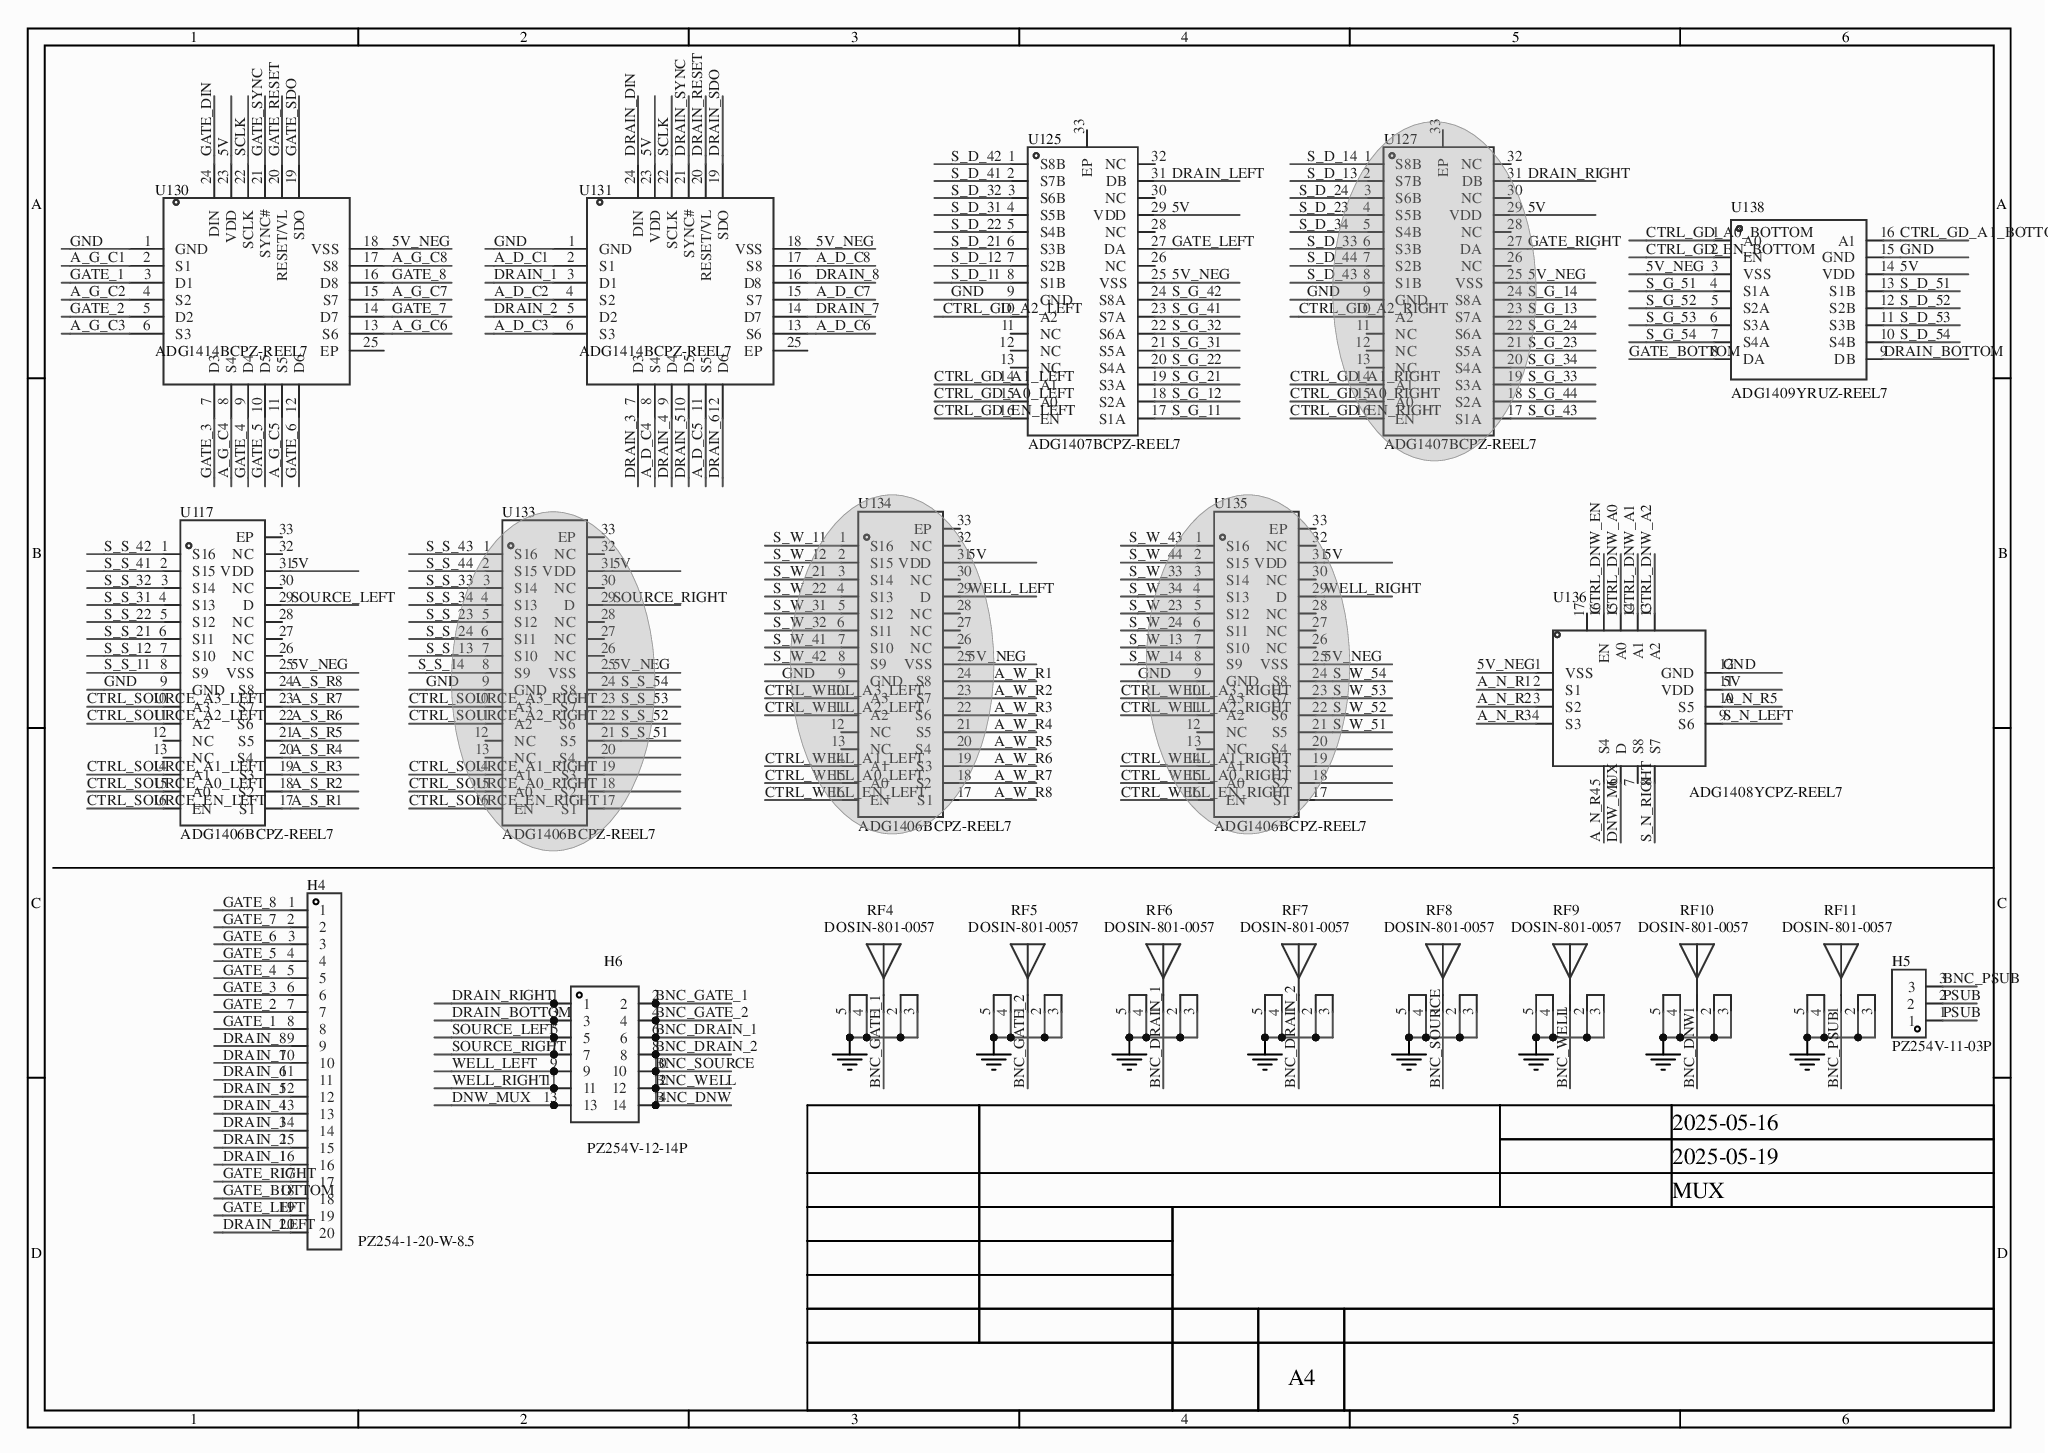
[diagram p0: MISC82799-4.schdoc]
# Altium project MISC82799-9.PrjPCB (part 3 of 3)

## Nets that join several sheets
GND: MISC82799-2 (71 pins), MISC82799-4 (42 pins)
5V: MISC82799-2 (17 pins), MISC82799-4 (10 pins)
5V_NEG: MISC82799-2 (6 pins), MISC82799-4 (10 pins)
A_D_C1: MISC82799-2 (U4.16), MISC82799-4 (U131.2)
A_D_C2: MISC82799-2 (U4.19), MISC82799-4 (U131.4)
A_D_C3: MISC82799-2 (U4.17), MISC82799-4 (U131.6)
A_D_C4: MISC82799-2 (U4.20), MISC82799-4 (U131.8)
A_D_C5: MISC82799-2 (U5.18), MISC82799-4 (U131.11)
A_D_C6: MISC82799-2 (U5.19), MISC82799-4 (U131.13)
A_D_C7: MISC82799-2 (U5.15), MISC82799-4 (U131.15)
A_D_C8: MISC82799-2 (U5.20), MISC82799-4 (U131.17)
A_G_C1: MISC82799-2 (U4.1), MISC82799-4 (U130.2)
A_G_C2: MISC82799-2 (U4.5), MISC82799-4 (U130.4)
A_G_C3: MISC82799-2 (U4.2), MISC82799-4 (U130.6)
A_G_C4: MISC82799-2 (U4.6), MISC82799-4 (U130.8)
A_G_C5: MISC82799-2 (U5.1), MISC82799-4 (U130.11)
A_G_C6: MISC82799-2 (U5.5), MISC82799-4 (U130.13)
A_G_C7: MISC82799-2 (U5.2), MISC82799-4 (U130.15)
A_G_C8: MISC82799-2 (U5.6), MISC82799-4 (U130.17)
A_N_R1: MISC82799-2 (U4.4), MISC82799-4 (U136.2)
A_N_R2: MISC82799-2 (U4.3), MISC82799-4 (U136.3)
A_N_R3: MISC82799-2 (U5.3), MISC82799-4 (U136.4)
A_N_R4: MISC82799-2 (U5.4), MISC82799-4 (U136.5)
A_N_R5: MISC82799-2 (U4.15), MISC82799-4 (U136.10)
A_S_R1: MISC82799-2 (U4.8), MISC82799-4 (U117.17)
A_S_R2: MISC82799-2 (U4.7), MISC82799-4 (U117.18)
A_S_R3: MISC82799-2 (U4.10), MISC82799-4 (U117.19)
A_S_R4: MISC82799-2 (U4.9), MISC82799-4 (U117.20)
A_S_R5: MISC82799-2 (U4.12), MISC82799-4 (U117.21)
A_S_R6: MISC82799-2 (U4.11), MISC82799-4 (U117.22)
A_S_R7: MISC82799-2 (U4.14), MISC82799-4 (U117.23)
A_S_R8: MISC82799-2 (U4.13), MISC82799-4 (U117.24)
A_W_R1: MISC82799-2 (U5.7), MISC82799-4 (U134.24)
A_W_R2: MISC82799-2 (U5.8), MISC82799-4 (U134.23)
A_W_R3: MISC82799-2 (U5.9), MISC82799-4 (U134.22)
A_W_R4: MISC82799-2 (U5.10), MISC82799-4 (U134.21)
A_W_R5: MISC82799-2 (U5.11), MISC82799-4 (U134.20)
A_W_R6: MISC82799-2 (U5.12), MISC82799-4 (U134.19)
A_W_R7: MISC82799-2 (U5.13), MISC82799-4 (U134.18)
A_W_R8: MISC82799-2 (U5.14), MISC82799-4 (U134.17)
CTRL_DNW_A0: MISC82799-2 (FPGAJ4.9 H3.9), MISC82799-4 (U136.15)
CTRL_DNW_A1: MISC82799-2 (FPGAJ4.8 H3.10), MISC82799-4 (U136.14)
CTRL_DNW_A2: MISC82799-2 (FPGAJ4.7 H3.11), MISC82799-4 (U136.13)
CTRL_DNW_EN: MISC82799-2 (FPGAJ4.10 H3.8), MISC82799-4 (U136.16)
CTRL_GD_A0_BOTTOM: MISC82799-2 (FPGAJ2.15 H2.13), MISC82799-4 (U138.1)
CTRL_GD_A0_LEFT: MISC82799-2 (FPGAJ2.19 H2.17), MISC82799-4 (U125.15)
CTRL_GD_A0_RIGHT: MISC82799-2 (FPGAJ2.4 H2.2), MISC82799-4 (U127.15)
CTRL_GD_A1_BOTTOM: MISC82799-2 (FPGAJ2.17 H2.15), MISC82799-4 (U138.16)
CTRL_GD_A1_LEFT: MISC82799-2 (FPGAJ2.20 H2.18), MISC82799-4 (U125.14)
CTRL_GD_A1_RIGHT: MISC82799-2 (FPGAJ2.5 H2.3), MISC82799-4 (U127.14)
CTRL_GD_A2_LEFT: MISC82799-2 (FPGAJ2.18 H2.16), MISC82799-4 (U125.10)
CTRL_GD_A2_RIGHT: MISC82799-2 (FPGAJ2.6 H2.4), MISC82799-4 (U127.10)
CTRL_GD_EN_BOTTOM: MISC82799-2 (FPGAJ2.16 H2.14), MISC82799-4 (U138.2)
CTRL_GD_EN_LEFT: MISC82799-2 (FPGAJ2.22 H2.20), MISC82799-4 (U125.16)
CTRL_GD_EN_RIGHT: MISC82799-2 (FPGAJ2.3 H2.1), MISC82799-4 (U127.16)
CTRL_SOURCE_A0_LEFT: MISC82799-2 (FPGAJ2.26 H2.24), MISC82799-4 (U117.15)
CTRL_SOURCE_A0_RIGHT: MISC82799-2 (FPGAJ2.30 H2.28), MISC82799-4 (U133.15)
CTRL_SOURCE_A1_LEFT: MISC82799-2 (FPGAJ2.23 H2.21), MISC82799-4 (U117.14)
CTRL_SOURCE_A1_RIGHT: MISC82799-2 (FPGAJ2.31 H2.29), MISC82799-4 (U133.14)
CTRL_SOURCE_A2_LEFT: MISC82799-2 (FPGAJ2.24 H2.22), MISC82799-4 (U117.11)
CTRL_SOURCE_A2_RIGHT: MISC82799-2 (FPGAJ2.32 H2.30), MISC82799-4 (U133.11)
CTRL_SOURCE_A3_LEFT: MISC82799-2 (FPGAJ2.21 H2.19), MISC82799-4 (U117.10)
CTRL_SOURCE_A3_RIGHT: MISC82799-2 (FPGAJ2.33 H2.31), MISC82799-4 (U133.10)
CTRL_SOURCE_EN_LEFT: MISC82799-2 (FPGAJ2.25 H2.23), MISC82799-4 (U117.16)
CTRL_SOURCE_EN_RIGHT: MISC82799-2 (FPGAJ2.29 H2.27), MISC82799-4 (U133.16)
CTRL_WELL_A0_LEFT: MISC82799-2 (FPGAJ2.35 H2.33), MISC82799-4 (U134.15)
CTRL_WELL_A0_RIGHT: MISC82799-2 (FPGAJ4.14 H3.4), MISC82799-4 (U135.15)
CTRL_WELL_A1_LEFT: MISC82799-2 (FPGAJ2.36 H2.34), MISC82799-4 (U134.14)
CTRL_WELL_A1_RIGHT: MISC82799-2 (FPGAJ4.13 H3.5), MISC82799-4 (U135.14)
CTRL_WELL_A2_LEFT: MISC82799-2 (FPGAJ2.27 H2.25), MISC82799-4 (U134.11)
CTRL_WELL_A2_RIGHT: MISC82799-2 (FPGAJ4.12 H3.6), MISC82799-4 (U135.11)
CTRL_WELL_A3_LEFT: MISC82799-2 (FPGAJ2.28 H2.26), MISC82799-4 (U134.10)
CTRL_WELL_A3_RIGHT: MISC82799-2 (FPGAJ4.11 H3.7), MISC82799-4 (U135.10)
CTRL_WELL_EN_LEFT: MISC82799-2 (FPGAJ2.34 H2.32), MISC82799-4 (U134.16)
CTRL_WELL_EN_RIGHT: MISC82799-2 (FPGAJ4.15 H3.3), MISC82799-4 (U135.16)
DRAIN_DIN: MISC82799-2 (FPGAJ2.7 H2.5), MISC82799-4 (U131.24)
DRAIN_RESET: MISC82799-2 (FPGAJ2.9 H2.7), MISC82799-4 (U131.20)
DRAIN_SDO: MISC82799-2 (FPGAJ2.10 H2.8), MISC82799-4 (U131.19)
DRAIN_SYNC: MISC82799-2 (FPGAJ2.8 H2.6), MISC82799-4 (U131.21)
GATE_DIN: MISC82799-2 (FPGAJ2.11 H2.9), MISC82799-4 (U130.24)
GATE_RESET: MISC82799-2 (FPGAJ2.13 H2.11), MISC82799-4 (U130.20)
GATE_SDO: MISC82799-2 (FPGAJ2.14 H2.12), MISC82799-4 (U130.19)
GATE_SYNC: MISC82799-2 (FPGAJ2.12 H2.10), MISC82799-4 (U130.21)
PSUB: MISC82799-2 (U5.16), MISC82799-4 (H5.1 H5.2)
S_D_11: MISC82799-2 (U4.26), MISC82799-4 (U125.8)
S_D_12: MISC82799-2 (U4.28), MISC82799-4 (U125.7)
S_D_13: MISC82799-2 (U5.28), MISC82799-4 (U127.2)
S_D_14: MISC82799-2 (U5.26), MISC82799-4 (U127.1)
S_D_21: MISC82799-2 (U4.34), MISC82799-4 (U125.6)
S_D_22: MISC82799-2 (U4.36), MISC82799-4 (U125.5)
S_D_23: MISC82799-2 (U5.36), MISC82799-4 (U127.4)
S_D_24: MISC82799-2 (U5.34), MISC82799-4 (U127.3)
S_D_31: MISC82799-2 (U4.41), MISC82799-4 (U125.4)
S_D_32: MISC82799-2 (U4.43), MISC82799-4 (U125.3)
S_D_33: MISC82799-2 (U5.44), MISC82799-4 (U127.6)
S_D_34: MISC82799-2 (U5.42), MISC82799-4 (U127.5)
S_D_41: MISC82799-2 (U4.50), MISC82799-4 (U125.2)
S_D_42: MISC82799-2 (U4.52), MISC82799-4 (U125.1)
S_D_43: MISC82799-2 (U5.52), MISC82799-4 (U127.8)
S_D_44: MISC82799-2 (U5.50), MISC82799-4 (U127.7)
S_D_51: MISC82799-2 (U4.58), MISC82799-4 (U138.13)
S_D_52: MISC82799-2 (U4.60), MISC82799-4 (U138.12)
S_D_53: MISC82799-2 (U5.60), MISC82799-4 (U138.11)
S_D_54: MISC82799-2 (U5.58), MISC82799-4 (U138.10)
S_G_11: MISC82799-2 (U4.22), MISC82799-4 (U125.17)
S_G_12: MISC82799-2 (U4.24), MISC82799-4 (U125.18)
S_G_13: MISC82799-2 (U5.24), MISC82799-4 (U127.23)
S_G_14: MISC82799-2 (U5.22), MISC82799-4 (U127.24)
S_G_21: MISC82799-2 (U4.30), MISC82799-4 (U125.19)
S_G_22: MISC82799-2 (U4.32), MISC82799-4 (U125.20)
S_G_23: MISC82799-2 (U5.32), MISC82799-4 (U127.21)
S_G_24: MISC82799-2 (U5.30), MISC82799-4 (U127.22)
S_G_31: MISC82799-2 (U4.38), MISC82799-4 (U125.21)
S_G_32: MISC82799-2 (U4.40), MISC82799-4 (U125.22)
S_G_33: MISC82799-2 (U5.40), MISC82799-4 (U127.19)
S_G_34: MISC82799-2 (U5.38), MISC82799-4 (U127.20)
S_G_41: MISC82799-2 (U4.46), MISC82799-4 (U125.23)
S_G_42: MISC82799-2 (U4.48), MISC82799-4 (U125.24)
S_G_43: MISC82799-2 (U5.48), MISC82799-4 (U127.17)
S_G_44: MISC82799-2 (U5.46), MISC82799-4 (U127.18)
S_G_51: MISC82799-2 (U4.54), MISC82799-4 (U138.4)
S_G_52: MISC82799-2 (U4.56), MISC82799-4 (U138.5)
S_G_53: MISC82799-2 (U5.56), MISC82799-4 (U138.6)
S_G_54: MISC82799-2 (U5.54), MISC82799-4 (U138.7)
S_N_LEFT: MISC82799-2 (U4.18), MISC82799-4 (U136.9)
S_N_RIGHT: MISC82799-2 (U5.17), MISC82799-4 (U136.8)
S_S_11: MISC82799-2 (U4.25), MISC82799-4 (U117.8)
S_S_12: MISC82799-2 (U4.27), MISC82799-4 (U117.7)
S_S_13: MISC82799-2 (U5.27), MISC82799-4 (U133.7)
S_S_14: MISC82799-2 (U5.25), MISC82799-4 (U133.8)
S_S_21: MISC82799-2 (U4.33), MISC82799-4 (U117.6)
S_S_22: MISC82799-2 (U4.35), MISC82799-4 (U117.5)
S_S_23: MISC82799-2 (U5.35), MISC82799-4 (U133.5)
S_S_24: MISC82799-2 (U5.33), MISC82799-4 (U133.6)
S_S_31: MISC82799-2 (U4.42), MISC82799-4 (U117.4)
S_S_32: MISC82799-2 (U4.44), MISC82799-4 (U117.3)
S_S_33: MISC82799-2 (U5.43), MISC82799-4 (U133.3)
S_S_34: MISC82799-2 (U5.41), MISC82799-4 (U133.4)
S_S_41: MISC82799-2 (U4.49), MISC82799-4 (U117.2)
S_S_42: MISC82799-2 (U4.51), MISC82799-4 (U117.1)
S_S_43: MISC82799-2 (U5.51), MISC82799-4 (U133.1)
S_S_44: MISC82799-2 (U5.49), MISC82799-4 (U133.2)
S_S_51: MISC82799-2 (U4.57), MISC82799-4 (U133.21)
S_S_52: MISC82799-2 (U4.59), MISC82799-4 (U133.22)
S_S_53: MISC82799-2 (U5.59), MISC82799-4 (U133.23)
S_S_54: MISC82799-2 (U5.57), MISC82799-4 (U133.24)
S_W_11: MISC82799-2 (U4.21), MISC82799-4 (U134.1)
S_W_12: MISC82799-2 (U4.23), MISC82799-4 (U134.2)
S_W_13: MISC82799-2 (U5.23), MISC82799-4 (U135.7)
S_W_14: MISC82799-2 (U5.21), MISC82799-4 (U135.8)
S_W_21: MISC82799-2 (U4.29), MISC82799-4 (U134.3)
S_W_22: MISC82799-2 (U4.31), MISC82799-4 (U134.4)
S_W_23: MISC82799-2 (U5.31), MISC82799-4 (U135.5)
S_W_24: MISC82799-2 (U5.29), MISC82799-4 (U135.6)
S_W_31: MISC82799-2 (U4.37), MISC82799-4 (U134.5)
S_W_32: MISC82799-2 (U4.39), MISC82799-4 (U134.6)
S_W_33: MISC82799-2 (U5.39), MISC82799-4 (U135.3)
S_W_34: MISC82799-2 (U5.37), MISC82799-4 (U135.4)
S_W_41: MISC82799-2 (U4.45), MISC82799-4 (U134.7)
S_W_42: MISC82799-2 (U4.47), MISC82799-4 (U134.8)
S_W_43: MISC82799-2 (U5.47), MISC82799-4 (U135.1)
S_W_44: MISC82799-2 (U5.45), MISC82799-4 (U135.2)
S_W_51: MISC82799-2 (U4.53), MISC82799-4 (U135.21)
S_W_52: MISC82799-2 (U4.55), MISC82799-4 (U135.22)
S_W_53: MISC82799-2 (U5.55), MISC82799-4 (U135.23)
S_W_54: MISC82799-2 (U5.53), MISC82799-4 (U135.24)
SCLK: MISC82799-2 (FPGAJ4.16 H3.13 U96.13), MISC82799-4 (U130.22 U131.22)